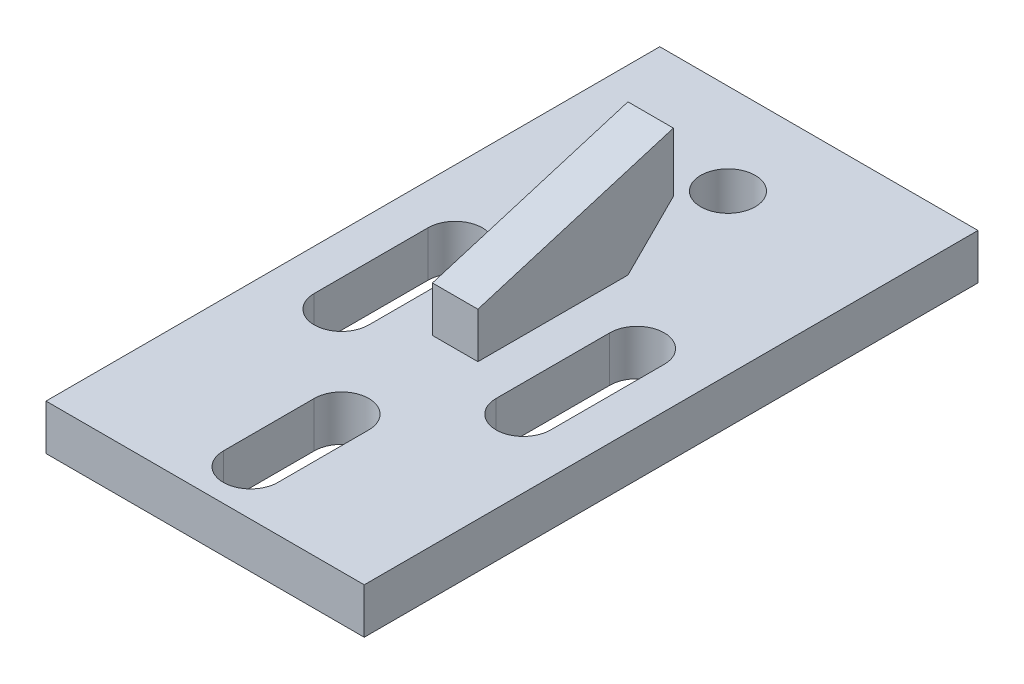
from build123d import *

# Parameters (mm, degrees)
SKETCH_1_W      = 70
SKETCH_1_H      = 135
SKETCH_1_R      = 6
EXTRUDE_1_DEPTH = 10
EXTRUDE_2_DEPTH = 5


with BuildPart() as part:
    # 草图1 → 凸台-拉伸1 (new body)
    with BuildSketch(Plane(origin=(0, 0, 0), x_dir=(1, 0, 0), z_dir=(0, 1, 0))):
        Rectangle(SKETCH_1_W, SKETCH_1_H)
        with Locations(Location((0, 47.5, 0), (0, 0, 270))):
            Circle(SKETCH_1_R, mode=Mode.SUBTRACT)
        with BuildLine():
            Line((6, -37.5), (6, -57.5))
            ThreePointArc((6, -57.5), (0, -63.5), (-6, -57.5))
            Line((-6, -57.5), (-6, -37.5))
            ThreePointArc((-6, -37.5), (0, -31.5), (6, -37.5))
        make_face(mode=Mode.SUBTRACT)
        with BuildLine():
            Line((-14, 7.5), (-14, -17.5))
            ThreePointArc((-14, -17.5), (-20, -23.5), (-26, -17.5))
            Line((-26, -17.5), (-26, 7.5))
            ThreePointArc((-26, 7.5), (-20, 13.5), (-14, 7.5))
        make_face(mode=Mode.SUBTRACT)
        with BuildLine():
            Line((14, 7.5), (14, -17.5))
            ThreePointArc((14, -17.5), (20, -23.5), (26, -17.5))
            Line((26, -17.5), (26, 7.5))
            ThreePointArc((26, 7.5), (20, 13.5), (14, 7.5))
        make_face(mode=Mode.SUBTRACT)
    extrude(amount=EXTRUDE_1_DEPTH)


with BuildPart() as body_2:
    # 草图2 → 凸台-拉伸2 (new, symmetric)
    with BuildSketch(Plane(origin=(0, 0, 0), x_dir=(0, 0, -1), z_dir=(1, 0, 0))):
        Polygon((-12.5, 10), (-12.5, 20), (30.5, 33), (30.5, 20), (20.5, 10), align=None)
    extrude(amount=EXTRUDE_2_DEPTH, both=True)


solid = Compound([part.part, body_2.part])
